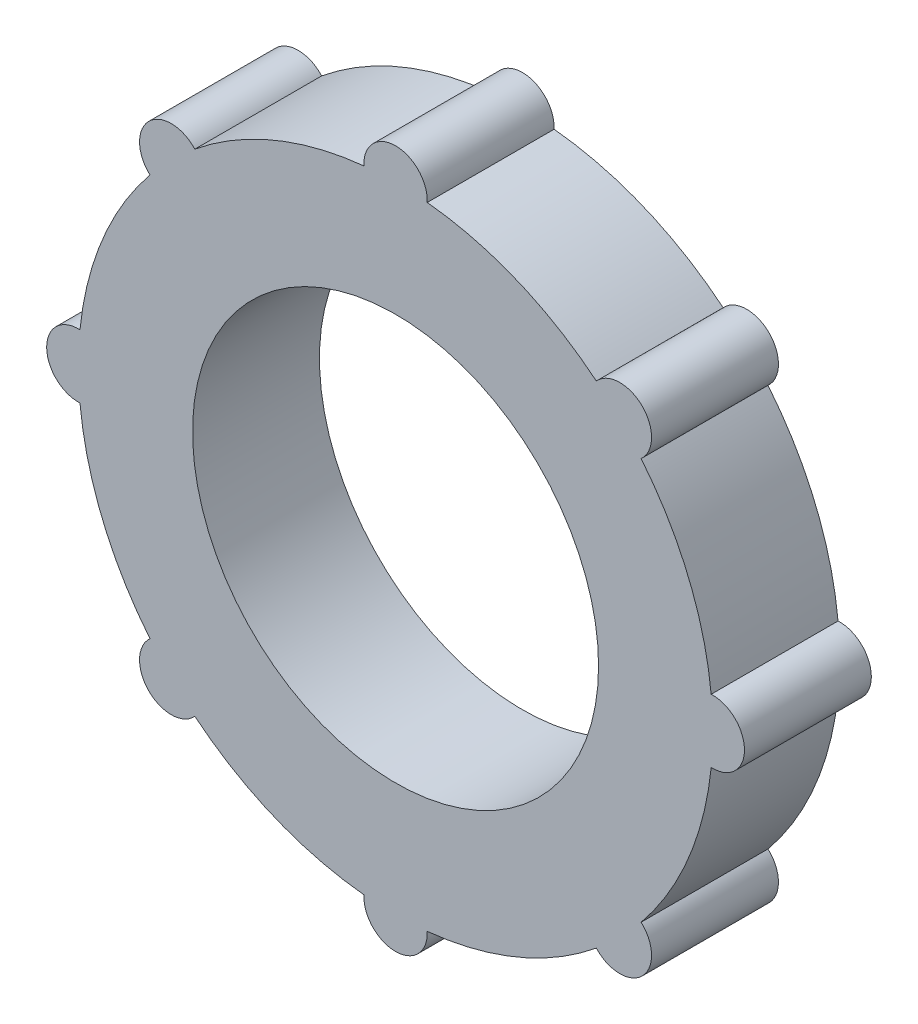
from build123d import *

# Parameters (mm, degrees)
SKETCH_1_R      = 16
EXTRUDE_1_DEPTH = 10


with BuildPart() as part:
    # 草图1 → 凸台-拉伸1 (new body)
    with BuildSketch(Plane.XY):
        with BuildLine():
            ThreePointArc((-2.496873044, 24.875), (-9.567085809, 23.096988313), (-15.823725321, 19.354837043))
            ThreePointArc((-15.823725321, 19.354837043), (-19.445436483, 19.445436483), (-19.354837043, 15.823725321))
            ThreePointArc((-19.354837043, 15.823725321), (-23.096988313, 9.567085809), (-24.875, 2.496873044))
            ThreePointArc((-24.875, 2.496873044), (-27.5, 0), (-24.875, -2.496873044))
            ThreePointArc((-24.875, -2.496873044), (-23.096988313, -9.567085809), (-19.354837043, -15.823725321))
            ThreePointArc((-19.354837043, -15.823725321), (-19.445436483, -19.445436483), (-15.823725321, -19.354837043))
            ThreePointArc((-15.823725321, -19.354837043), (-9.567085809, -23.096988313), (-2.496873044, -24.875))
            ThreePointArc((-2.496873044, -24.875), (0, -27.5), (2.496873044, -24.875))
            ThreePointArc((2.496873044, -24.875), (9.567085809, -23.096988313), (15.823725321, -19.354837043))
            ThreePointArc((15.823725321, -19.354837043), (19.445436483, -19.445436483), (19.354837043, -15.823725321))
            ThreePointArc((19.354837043, -15.823725321), (23.096988313, -9.567085809), (24.875, -2.496873044))
            ThreePointArc((24.875, -2.496873044), (27.5, 0), (24.875, 2.496873044))
            ThreePointArc((24.875, 2.496873044), (23.096988313, 9.567085809), (19.354837043, 15.823725321))
            ThreePointArc((19.354837043, 15.823725321), (19.445436483, 19.445436483), (15.823725321, 19.354837043))
            ThreePointArc((15.823725321, 19.354837043), (9.567085809, 23.096988313), (2.496873044, 24.875))
            ThreePointArc((2.496873044, 24.875), (0, 27.5), (-2.496873044, 24.875))
        make_face()
        Circle(SKETCH_1_R, mode=Mode.SUBTRACT)
    extrude(amount=EXTRUDE_1_DEPTH)


solid = part.part
